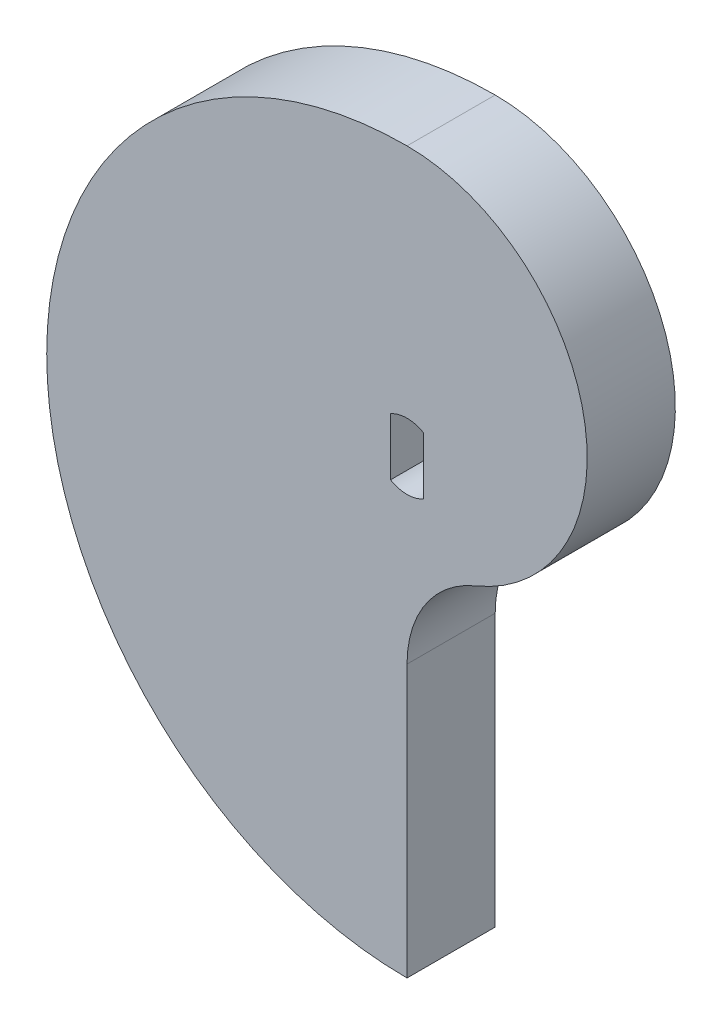
from build123d import *

# Parameters (mm, degrees)
SKETCH4_R           = 2.5
BOSS_EXTRUDE3_DEPTH = 4
FILLET2_R           = 5
SKETCH7_R           = 3.986171954
SKETCH7_R_2         = 1.5
BOSS_EXTRUDE4_DEPTH = 4
BOSS_EXTRUDE5_DEPTH = 4
SKETCH9_R           = 1.5
CUT_EXTRUDE1_DEPTH  = 27.524941093
BOSS_EXTRUDE6_DEPTH = 4


with BuildPart() as part:
    # Sketch4 → Boss-Extrude3 (new body)
    with BuildSketch(Plane.XY):
        with BuildLine():
            Line((0, -20.5), (0, -4.15))
            ThreePointArc((0, -4.15), (8.175, 4.025), (0, 12.2))
            ThreePointArc((0, 12.2), (-16.35, -4.15), (0, -20.5))
        make_face()
        Circle(SKETCH4_R, mode=Mode.SUBTRACT)
    extrude(amount=BOSS_EXTRUDE3_DEPTH)

    # Fillet2
    fillet2_edges = [part.edges().sort_by_distance(p)[0] for p in [
        (0, -4.15, 2),
    ]]
    fillet(fillet2_edges, radius=FILLET2_R)

    # Sketch7 → Boss-Extrude4 (add)
    with BuildSketch(Plane.XY.offset(4)):
        Circle(SKETCH7_R)
        Circle(SKETCH7_R_2, mode=Mode.SUBTRACT)
    extrude(amount=-BOSS_EXTRUDE4_DEPTH)

    # Sketch8 → Boss-Extrude5 (add)
    with BuildSketch(Plane.XY.offset(4)):
        Polygon((0, 0), (-1, 1.118033989), (-1.075164003, 1.990831029), (0.996128458, 2.028687549), (1.118033989, 1), align=None)
    extrude(amount=-BOSS_EXTRUDE5_DEPTH)

    # Sketch9 → Cut-Extrude1 (cut, through all)
    with BuildSketch(Plane.XY.offset(4)):
        Circle(SKETCH9_R)
    extrude(amount=-CUT_EXTRUDE1_DEPTH, mode=Mode.SUBTRACT)

    # Sketch10 → Boss-Extrude6 (add, through all)
    with BuildSketch(Plane.XY.offset(4)):
        with BuildLine():
            ThreePointArc((1.5, 0), (1.299038106, 0.75), (0.75, 1.299038106))
            Line((0.75, 1.299038106), (0.75, -1.299038106))
            ThreePointArc((0.75, -1.299038106), (1.299038106, -0.75), (1.5, 0))
        make_face()
        with BuildLine():
            Line((-0.75, -1.299038106), (-0.75, 1.299038106))
            ThreePointArc((-0.75, 1.299038106), (-1.5, 0), (-0.75, -1.299038106))
        make_face()
    extrude(amount=-BOSS_EXTRUDE6_DEPTH)


solid = part.part
